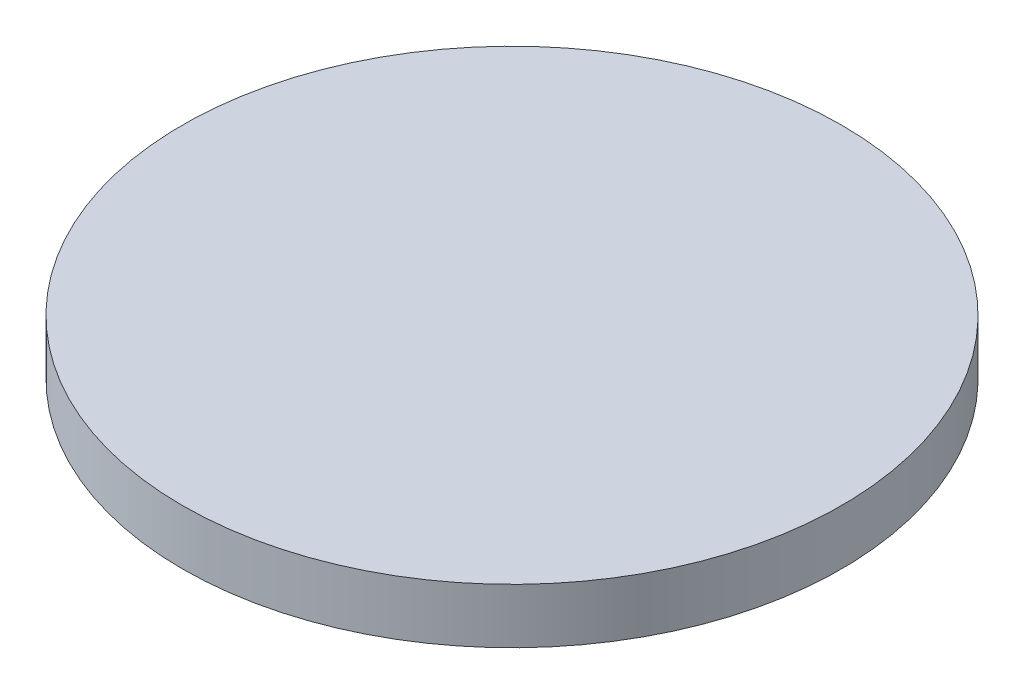
from build123d import *

# Parameters (mm, degrees)
SKETCH1_R           = 30
BOSS_EXTRUDE1_DEPTH = 5


with BuildPart() as part:
    # Sketch1 → Boss-Extrude1 (new body)
    with BuildSketch(Plane(origin=(0, 0, 0), x_dir=(1, 0, 0), z_dir=(0, 1, 0))):
        with Locations(Location((0, 0, 0), (0, 0, 270))):
            Circle(SKETCH1_R)
    extrude(amount=BOSS_EXTRUDE1_DEPTH)


solid = part.part
